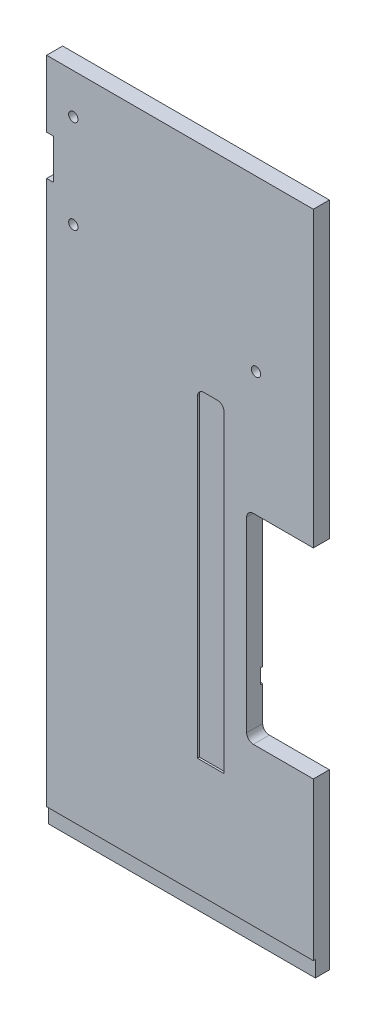
SolidWorks part; units mm, degrees
ref_plane "前视基准面" through (0, 0, 0) normal (0, 0, 1) x (1, 0, 0)
ref_plane "上视基准面" through (0, 0, 0) normal (0, 1, 0) x (1, 0, 0)
ref_plane "右视基准面" through (0, 0, 0) normal (1, 0, 0) x (0, 0, -1)
sketch "草图1" plane through (0, 0, 0) normal (0, 0, 1) x (1, 0, 0)
  line L1 (-100, -250) -> (100, -250)
  line L2 (-100, -250) -> (-100, 250)
  line L3 (-100, 250) -> (100, 250)
  line L4 (100, -250) -> (100, 250)
  line L5 (-100, -250) -> (100, 250) construction
  line L6 (-100, 250) -> (100, -250) construction
  point P0 (0, 0)
  dimension "D1" = 200
  dimension "D2" = 500
extrude "凸台-拉伸1" add sketch "草图1" along normal mid plane 12
sketch "草图2" plane through (0, 0, -6) normal (0, 0, 1) x (1, 0, 0)
  line L0 (-100, 250) -> (-100, -250) construction
  line L1 (-100, -89) -> (100, -89)
  line L2 (-100, -89) -> (-100, -78)
  line L3 (-100, -78) -> (100, -78)
  line L4 (100, -89) -> (100, -78)
  line L5 (100, -250) -> (100, 250) construction
  line L6 (-100, -250) -> (100, -250) construction
  dimension "D1" = 11
  dimension "D2" = 161
extrude "切除-拉伸1" cut sketch "草图2" along normal blind 1.5
sketch "草图3" plane through (0, 0, 6) normal (0, 0, 1) x (1, 0, 0)
  line L0 (-95, 200) -> (-100, 200)
  line L2 (-100, 200) -> (-100, 170)
  line L3 (-100, 170) -> (-95, 170)
  line L4 (-95, 170) -> (-95, 200)
  line L5 (100, 250) -> (-100, 250) construction
  line L6 (-100, 250) -> (-100, -250) construction
  point P2 (-100.6065, 200)
  point P3 (0, 0)
  point P8 (0, 0)
  dimension "D1" = 5
  dimension "D2" = 30
  dimension "D3" = 50
extrude "切除-拉伸2" cut sketch "草图3" against normal up to next
sketch "草图4" plane through (0, 0, 6) normal (0, 0, 1) x (1, 0, 0)
  line L0 (-100, 250) -> (-100, 200) construction
  line L1 (-95, 200) -> (-100, 200) construction
  line L2 (-100, 170) -> (-95, 170) construction
  line L3 (-80, 136.5) -> (57, 136.5) construction
  line L4 (100, -250) -> (100, 250) construction
  circle A0 centre (-80, 220) radius 3.5
  circle A1 centre (-80, 150) radius 3.5
  circle A2 centre (57, 123) radius 3.5
  circle A3 centre (-80, 150) radius 13.5 construction
  circle A4 centre (57, 123) radius 13.5 construction
extrude "切除-拉伸3" cut sketch "草图4" against normal up to next
sketch "草图5" plane through (0, 0, 6) normal (0, 0, -1) x (-1, 0, 0)
  line L1 (-33, -150) -> (-13, -150)
  line L2 (-33, -150) -> (-33, 90)
  line L3 (-33, 90) -> (-13, 90)
  line L4 (-13, -150) -> (-13, 90)
  line L5 (-100, -250) -> (-100, -89) construction
  line L6 (100, -250) -> (-100, -250) construction
  dimension "D1" = 20
  dimension "D2" = 240
  dimension "D3" = 67
  dimension "D4" = 100
extrude "切除-拉伸4" cut sketch "草图5" along normal blind 1.5
fillet "圆角1" radius 5 2 edges at (13, 90, 5.25) (33, 90, 5.25)
sketch "草图6" plane through (0, 0, -6) normal (0, 0, -1) x (-1, 0, 0)
  line L0 (-100, -250) -> (-100, -89) construction
  line L1 (-100, -120) -> (-50, -120)
  line L2 (-100, -120) -> (-100, 30)
  line L3 (-100, 30) -> (-50, 30)
  line L4 (-50, -120) -> (-50, 30)
  line L5 (100, -250) -> (-100, -250) construction
  point P12 (0, -250)
  dimension "D1" = 150
  dimension "D2" = 50
  dimension "D3" = 130
extrude "切除-拉伸5" cut sketch "草图6" against normal up to next
fillet "圆角2" radius 5 2 edges at (50, 30, 0) (50, -120, 0)
sketch "草图7" plane through (0, 0, 6) normal (0, 0, 1) x (1, 0, 0)
  line L0 (100, -250) -> (100, -120) construction
  line L1 (-100, -250) -> (100, -250)
  line L2 (-100, -250) -> (-100, -238)
  line L3 (-100, -238) -> (100, -238)
  line L4 (100, -250) -> (100, -238)
  dimension "D1" = 12
extrude "切除-拉伸6" cut sketch "草图7" against normal blind 1.5
equation "\"D4@草图4\"=\"D3@草图4\""
